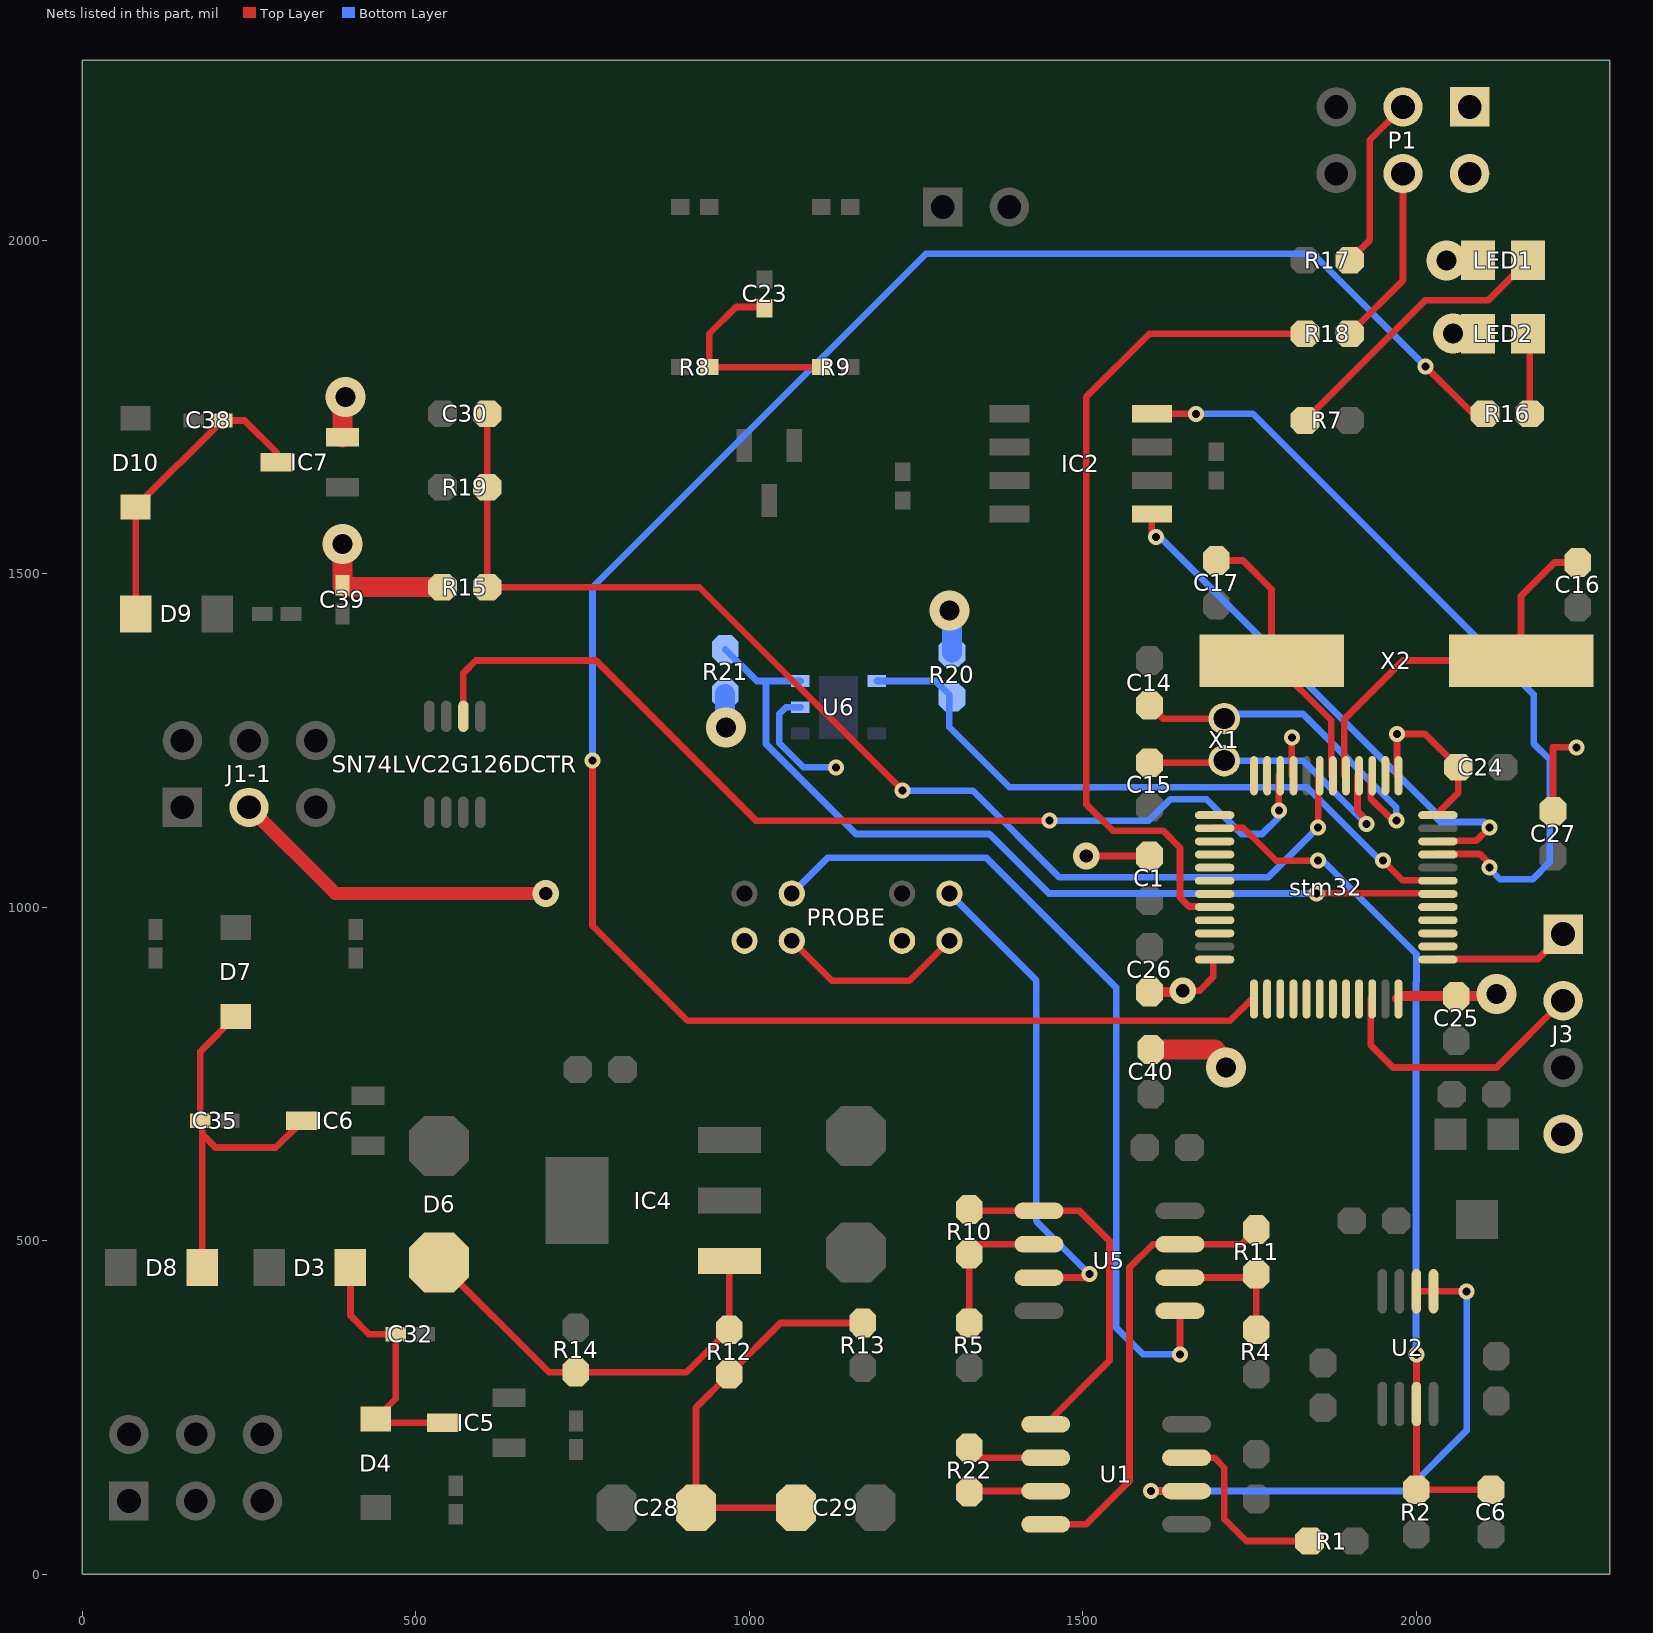
[diagram p0: the nets of this part, all layers, seen from the top]
# Altium PCB MISC82170.PcbDoc (part 2 of 2)
Units mil, origin at the board's own origin, x right, y up, seen from the top; angles counter-clockwise.
Board outline 2290 x 2270 mil, 4 copper layers (Top Layer, GND, VCC, Bottom Layer), stack 43.156 mil thick; 86 components, 73 nets, 279 pads, 92 vias.

## Via types
v1: diameter 60, hole 30, Top Layer to Bottom Layer, 42 vias
v2: diameter 24, hole 12, Top Layer to Bottom Layer, 34 vias
v3: diameter 40, hole 20, Top Layer to Bottom Layer, 16 vias

## Nets (pads, with @x,y where several pads share a name; then routed paths per layer and width w, separated by ;. In a path a pad name is that pad's centre, name@x,y a point inside that pad or via, vN(x,y) a via of type N, cw(c..) or ccw(c..) an arc to the next point about the centre after c; other vN are vias at no path point) (continued)
NetC23_1: C23.1 R8.2 R9.1 | length 318.3
  Top Layer w10: C23.1@1022.89,1898.03 1020.92,1900 980,1900 940,1860 R8.2@940,1810 R9.1@1108.03,1810
NetC28_2: C28.2 C29.2 R12.1 R13.2 | length 602.6
  Top Layer w10: C29.2@1070,100 C28.2@920,100 920,250 R12.1@970,300 1047,377 R13.2@1170,377
NetC32_2: C32.2 D3.2 D4.2 IC5.3 | length 394.8
  Top Layer w10: D3.2@402.05,460 402.05,387.95 430,360 C32.2@470,360 470,263.26 D4.2@440,233.26 445.86,227.4 IC5.3@541.6,227.4
NetC35_2: C35.2 D7.2 D8.2 IC6.3 | length 574.7
  Top Layer w10: D8.2@180,460 180,660 ; D7.2@230,836.74 177.08,783.82 C35.2@177.08,680 180,677.08 180,660 ; IC6.3@330,680 290,640 200,640 180,660
NetC38_2: C38.2 D9.2 D10.2 IC7.3 | length 459.8
  Top Layer w10: D9.2@80,1440 D10.2@80,1600 C38.2@210,1730 243.31,1730 291.6,1681.71 IC7.3@291.6,1667.4
NetD6_1: D6.1 IC4.1 R12.2 R14.1 | length 632.6
  Top Layer w10: D6.1@535,467.5 699.5,303 R14.1@740,303 906,303 R12.2@970,367 IC4.1@970,470
NetLED1_2: LED1.2 R7.1 | length 433.8
  Top Layer w10: R7.1@1833,1730 2013,1910 2107.4,1910 LED1.2@2167.4,1970
NetLED2_2: LED2.2 R16.1 | length 121.1
  Top Layer w10: LED2.2@2167.4,1860 2170,1857.4 R16.1@2170,1740
NetP1_3: P1.3 R17.2 | length 263.1
  Top Layer w10: R17.2@1900,1970 1930,2000 1930,2150 P1.3@1980,2200
NetP1_4: P1.4 R18.2 | length 273.1
  Top Layer w10: R18.2@1900,1860 1980,1940 P1.4@1980,2100
NetPROBE_V1-: PROBE.2 PROBE.6 | length 285.9
  Top Layer w10: PROBE.2@1063.78,950 1123.78,890 1240,890 PROBE.6@1300,950
NetPROBE_V+/V2+: PROBE.5 U5.3 | length 735.5
  Top Layer w10: U5.3@1434.39,445 1505,445 v2(1510,450)
  Bottom Layer w10: PROBE.5@1300,1020.87 1430,890.87 1430,530 v2(1510,450)
NetPROBE_V-/V1+: PROBE.1 U5.5 | length 1275.9
  Top Layer w10: v2(1645.61,330) U5.5@1645.61,395
  Bottom Layer w10: PROBE.1@1063.78,1020.87 1117.13,1074.22 1355.78,1074.22 1550,880 1550,370 1590,330 v2(1645.61,330)
NetR1_1: R1.1 U1.7 | length 281.3
  Top Layer w10: U1.7@1655.61,175 1697.07,175 1712.07,160 1712.07,82.93 1745,50 R1.1@1840,50
NetR4_2: R4.2 R11.2 U5.6 | length 199.5
  Top Layer w10: U5.6@1645.61,445 1755,445 R11.2@1760,450 R4.2@1760,367
NetR5_1: R5.1 R10.2 U5.2 | length 213.6
  Top Layer w10: R5.1@1330,377 R10.2@1330,480 1345,495 U5.2@1434.39,495
NetR10_1: R10.1 U1.1 U5.1 | length 544.1
  Top Layer w10: R10.1@1330,547 1332,545 U5.1@1434.39,545 1495,545 1540,500 1540,320.61 U1.1@1444.39,225
NetR11_1: R11.1 U1.4 U5.7 | length 686.1
  Top Layer w10: U1.4@1444.39,75 1505,75 1570,140 1570,460 1605,495 U5.7@1645.61,495 1738,495 R11.1@1760,517
NetR22_1: R22.1 U1.3 | length 115.2
  Top Layer w10: R22.1@1330,123 1332,125 U1.3@1444.39,125
NetR22_2: R22.2 U1.2 | length 120.6
  Top Layer w10: R22.2@1330,190 1345,175 U1.2@1444.39,175
NetU1_6: U1.6 U2.1 U2.2 | length 848.9
  Top Layer w10: v2(1602,125) U1.6@1655.61,125 ; U2.2@2000.19,424.49 U2.1@2025.79,424.49 v2(2075.51,424.49)
  Bottom Layer w10: v2(1602,125) 1985,125 2075.51,215.51 v2(2075.51,424.49)
NRST: C30.2 R15.1 R19.2 stm32.7 | length 1795.2
  Top Layer w10: C30.2@607,1740 R19.2@607,1630 R15.1@607,1480 925,1480 v2(1230,1175) ; v2(1852.84,1120) stm32.7@1852.84,1198.11
  Bottom Layer w10: v2(1230,1175) 1335,1175 1465,1045 1777.84,1045 v2(1852.84,1120)
OSC32_IN: C14.1 stm32.3 X1.1 | length 546.1
  Top Layer w10: C14.1@1600,1303 1620,1283 X1.1@1712.07,1283 ; stm32.3@1931.58,1198.11 1931.58,1163.42 1965,1130 v2(1970,1130)
  Bottom Layer w10: X1.1@1712.07,1283 1719.07,1290 1830,1290 1970,1150 v2(1970,1130)
OSC32_OUT: C15.1 stm32.4 X1.2 | length 444.1
  Top Layer w10: C15.1@1600,1217 1709.07,1217 X1.2@1712.07,1220 ; stm32.4@1911.89,1198.11 1911.89,1144.68 1925,1131.58 v2(1925,1125)
  Bottom Layer w10: X1.2@1712.07,1220 1830,1220 v2(1925,1125)
OSC_IN: C16.2 stm32.5 X2.1 | length 588
  Top Layer w10: stm32.5@1892.21,1198.11 1892.21,1282.21 1980,1370 X2.1@2157.01,1370 2157.01,1467.01 2207,1517 C16.2@2242,1517
OSC_OUT: C17.2 stm32.6 X2.2 | length 416.8
  Top Layer w10: C17.2@1700,1520 1740,1520 1782.99,1477.01 X2.2@1782.99,1370 1872.52,1280.47 stm32.6@1872.52,1198.11
PA0: SN74LVC2G126DCTR.2 stm32.10 | length 1502.8
  Top Layer w10: SN74LVC2G126DCTR.2@571.38,1286.38 571.38,1351.38 590,1370 770,1370 1010,1130 v2(1450,1130) ; v2(1793.78,1145) stm32.10@1793.78,1198.11
  Bottom Layer w10: v2(1450,1130) 1598.86,1130 1630.86,1162 1685.81,1162 1737.81,1110 1768.78,1110 1793.78,1135 v2(1793.78,1145)
PA1: stm32.11
PA2: stm32.12
PA3: stm32.13
PA4: C6.2 R2.2 stm32.14 U2.7 | length 1299.1
  Top Layer w10: stm32.14@1695.35,1119.37 1740.63,1119.37 1790,1070 v2(1852.84,1070) ; v2@2000,330 v2(2000.19,329.81) U2.7@2000.19,255.51 2000.19,127.19 R2.2@2000,127 C6.2@2112,127
  Bottom Layer w10: v2(1852.84,1070) 1860,1070 2000.19,929.81 2000.19,888.79 1999.5,888.11 1999.5,330.5 v2(2000.19,329.81)
PA5: stm32.15
PA6: stm32.16
PA7: stm32.17
PA8: stm32.29
PA9: stm32.30
PA10: stm32.31
PA15: stm32.38
PB0: stm32.18
PB1: stm32.19
PB2/BOOT1: R18.1 stm32.20 | length 1275
  Top Layer w10: stm32.20@1695.35,1001.26 1659.35,1001.26 1645.61,1015 1645.61,1089.39 1620,1115 1545,1115 1505,1155 1505,1765 1600,1860 R18.1@1833,1860
PB3: stm32.39
PB4: stm32.40
PB5: stm32.41
PB6: R21.1 stm32.42 U6.6 | length 1324.9
  Top Layer w10: v2(1850,1020.87) 1850.08,1020.94 stm32.42@2030,1020.94
  Bottom Layer w10: R21.1@963.78,1387 1011.41,1339.37 1025,1339.37 ; U6.6@1076.67,1339.37 1025,1339.37 ; v2(1850,1020.87) 1449.13,1020.87 1360,1110 1160,1110 1025,1245 1025,1339.37
PB7: R20.1 stm32.43 U6.1 | length 991.4
  Top Layer w10: v2(1950,1070) 1979.37,1040.63 stm32.43@2030,1040.63
  Bottom Layer w10: U6.1@1190.89,1339.37 1279.38,1339.37 1300,1318.75 1300,1270 1390,1180 1836.06,1180 1946.06,1070 v2(1950,1070)
PB8/CANRX: IC2.4 stm32.45 | length 1208.7
  Top Layer w10: IC2.4@1603.54,1740 v2(1670,1740) ; stm32.45@2030,1080 2095.31,1080 2110,1065.31 v2(2110,1060)
  Bottom Layer w10: v2(1670,1740) 1755,1740 2175.9,1319.1 2175.9,1245.89 2200,1221.79 2200,1067.89 2174.14,1042.03 2125.86,1042.03 2110,1057.89 v2(2110,1060)
PB9/CANTX: IC2.1 stm32.46 | length 830.5
  Top Layer w10: IC2.1@1603.54,1590 1603.54,1561.46 v2(1610,1555) ; stm32.46@2050,1100 2030.32,1100 2030,1099.68 2089.68,1099.68 v2(2110,1120)
  Bottom Layer w10: v2(1610,1555) 1615.93,1555 2030,1140.93 2030,1133.86 2035.86,1128 2102,1128 v2(2110,1120)
PB10: stm32.21
PB11: stm32.22
PB12: R16.2 stm32.25 | length 3215.3
  Top Layer w10: v2(765,1220) 765,972.52 907.52,830 1720.95,830 stm32.25@1754.41,863.46 ; v2(2014.01,1810.99) 2085,1740 R16.2@2103,1740
  Bottom Layer w10: v2(765,1220) 765,1480 1265,1980 1845,1980 v2(2014.01,1810.99) v2@2015,1810.99
PB13: stm32.26
PB14: stm32.27
PB15: stm32.28
PC13: stm32.2
SWCLK: J3.1 stm32.37 | length 205.5
  Top Layer w10: stm32.37@2030,922.52 2182.52,922.52 J3.1@2220,960
SWDIO: J3.2 stm32.34 | length 413.7
  Top Layer w10: stm32.34@1931.58,863.46 1931.58,793.42 1965,760 2120,760 J3.2@2220,860
USB_DM: stm32.32
USB_DP: stm32.33
VCC: C24.2 C25.2 C26.1 C27.1 C39.2 C40.2 IC7.2 J3.4 LED1.1 LED2.1 P1.1 P1.2 R15.2 R20.2 R21.2 stm32.1 stm32.9 stm32.24 stm32.36 stm32.48 U6.5 | length 1520.2
  Top Layer w10: v3(1650,875) 1675,875 1695.36,895.36 stm32.24@1695.36,922.52 ; stm32.9@1813.46,1198.11 v2(1813.46,1255) ; stm32.1@1970.95,1198.11 v2(1970.95,1260) 2013,1260 C24.2@2063,1210 2063,1172.05 stm32.48@2030,1139.05 ; C27.1@2205,1144 2205,1240 v2(2240,1240)
  Top Layer w15: C26.1@1600,873 1648,873 v3(1650,875) ; C40.2@1602,787 C40.2@1609,780 ; stm32.36@1970.95,863.46 1974.48,867 C25.2@2060,867 2117,867 v1(2120,870)
  Top Layer w30: v1@390,1540 C39.2@390,1482.92 392.92,1480 R15.2@540,1480 ; IC7.2@390,1704.8 390,1755 v1@395,1760 ; C40.2@1602,787 1698,787 1715,770 v1(1715,760) ; v1(2045,1970) LED1.1@2092.6,1970 ; v1@2053,1865 2058,1860 LED2.1@2092.6,1860
  Bottom Layer w10: U6.5@1076.67,1300 1055,1300 1045,1290 1045,1246.21 1081.21,1210 v2(1130,1210)
  Bottom Layer w30: R21.2@963.78,1320 963.78,1271.22 v1(965,1270) ; v1(1300,1445) 1303.78,1441.22 R20.2@1303.78,1381.97
  other v1: 390,1545 395,1765 2055,1860
Vin: C1.2 J1-1.3 PROBE.3 PROBE.7 | length 593.5
  Top Layer w10: v3(1505,1077) C1.2@1600,1077
  Top Layer w20: J1-1.3@250,1150 379.13,1020.87 v3(695,1020.87)
pads on no net: J1-1.2 J1-1.6 SN74LVC2G126DCTR.3 SN74LVC2G126DCTR.5 SN74LVC2G126DCTR.7 U6.3 U6.4

## Polygon pours and split planes (outlines as drawn)
GND on GND (split plane): 2269.9,20.1 20.1,20.1 20.1,30 20.1,2249.9 2269.9,2249.9
Vin on VCC (split plane): 1544.9,870.1 615.1,870.1 615.1,1124.9 1544.9,1124.9
2Vinput-2 on VCC (split plane): 604.9,705 605.29,703.05 606.4,701.4 608.05,700.29 610,699.9 944.9,699.9 944.9,355.1 740,355.1 738.05,354.71 736.4,353.6 735.29,351.95 734.9,350 734.9,184 735.29,182.05 736.4,180.4 738.05,179.29 740,178.9 741.95,179.29 742.87,179.9 885,179.9 886.95,180.29 888.6,181.4 889.71,183.05 890.1,185 890.1,229.9 1239.9,229.9 1239.9,155.1 630.1,155.1 630.1,270 630.1,505 629.71,506.95 628.6,508.6 626.95,509.71 625,510.1 312.07,510.1 311.82,510.05 308.61,509.8 305.23,508.98 305.1,508.93 305.1,689.9 510,689.9 511.95,690.29 513.6,691.4 514.71,693.05 515.1,695 515.1,830 514.71,831.95 513.6,833.6 511.95,834.71 510,835.1 415.1,835.1 415.1,1030 415.1,1200 414.71,1201.95 413.6,1203.6 411.95,1204.71 410,1205.1 305,1205.1 303.05,1204.71 301.4,1203.6 300.29,1201.95 299.9,1200 299.9,1035.1 200.1,1035.1 200.1,1314.9 604.9,1314.9
5V on VCC (split plane): 1884.9,1512.11 1781.4,1408.6 1746.4,1373.6 1745.29,1371.95 1744.9,1370 1744.9,1065 1745.29,1063.05 1746.4,1061.4 2004.9,802.89 2004.9,715 2005.29,713.05 2006.4,711.4 2051.4,666.4 2106.4,611.4 2108.05,610.29 2110,609.9 2269.9,609.9 2269.9,20.1 1325.1,20.1 1325.1,725 1324.71,726.95 1323.6,728.6 1321.95,729.71 1320,730.1 1120,730.1 1118.05,729.71 1116.4,728.6 1115.29,726.95 1114.9,725 1114.9,565 1115.29,563.05 1116.4,561.4 1118.05,560.29 1120,559.9 1239.9,559.9 1239.9,240.1 885,240.1 883.05,239.71 881.4,238.6 880.29,236.95 879.9,235 879.9,190.1 745.1,190.1 745.1,344.9 950,344.9 951.95,345.29 953.6,346.4 954.71,348.05 955.1,350 955.1,705 954.71,706.95 953.6,708.6 951.95,709.71 950,710.1 615.1,710.1 615.1,859.9 1429.83,859.9 1429.86,859.86 1431.51,858.75 1433.46,858.36 1435.41,858.75 1437.07,859.86 1437.11,859.9 1550,859.9 1551.95,860.29 1553.6,861.4 1554.71,863.05 1555.1,865 1555.1,1130 1554.71,1131.95 1553.6,1133.6 1551.95,1134.71 1550,1135.1 615.1,1135.1 615.1,1314.9 890.45,1314.9 890.45,1230 890.45,1180 890.84,1178.05 891.95,1176.4 893.6,1175.29 895.55,1174.9 1596.9,1174.9 1596.9,1136.69 1595.85,1134.72 1595.17,1132.49 1594.98,1130.58 1594.9,1130.17 1594.9,855 1594.9,850 1594.9,710 1594.9,706.04 1594.97,705.71 1595.2,703.38 1595.97,700.83 1597.23,698.48 1598.71,696.67 1598.9,696.4 1600.55,695.29 1602.5,694.9 1799.51,694.9 1801.46,695.29 1803.11,696.4 1804.22,698.05 1804.61,700 1804.61,702.89 1804.71,703.05 1805.1,705 1805.1,863.46 1804.71,865.41 1803.6,867.07 1744.96,925.72 1744.71,926.95 1743.6,928.6 1685.1,987.11 1685.1,1285 1684.71,1286.95 1683.6,1288.6 1418.6,1553.6 1416.95,1554.71 1415,1555.1 1175.1,1555.1 1175.1,1869.9 1884.9,1869.9
VCC on VCC (split plane): 2269.9,620.1 2112.11,620.1 2058.6,673.6 2015.1,717.11 2015.1,805 2014.71,806.95 2013.6,808.6 1755.1,1067.11 1755.1,1367.89 1788.6,1401.4 1893.6,1506.4 1894.71,1508.05 1895.1,1510 1895.1,1875 1894.71,1876.95 1893.6,1878.6 1891.95,1879.71 1890,1880.1 1170,1880.1 1168.05,1879.71 1166.4,1878.6 1165.29,1876.95 1164.9,1875 1164.9,1550 1165.29,1548.05 1166.4,1546.4 1168.05,1545.29 1170,1544.9 1412.89,1544.9 1674.9,1282.89 1674.9,985 1675.29,983.05 1676.4,981.4 1735.04,922.75 1735.29,921.51 1736.4,919.86 1794.9,861.35 1794.9,721.61 1794.8,721.46 1794.41,719.51 1794.41,705.1 1605.22,705.1 1605.07,705.87 1605.1,706.04 1605.1,710 1605.1,855 1605.1,1130.17 1605.08,1130.25 1605.2,1130.85 1605.54,1131.35 1605.6,1131.4 1606.71,1133.05 1607.1,1135 1607.1,1180 1606.71,1181.95 1605.6,1183.6 1603.95,1184.71 1602,1185.1 900.65,1185.1 900.65,1230 900.65,1318.67 900.54,1319.24 900.37,1320.46 899.68,1322.14 898.93,1323.12 898.6,1323.6 896.95,1324.71 895,1325.1 200.1,1325.1 200.1,1327.89 303.6,1431.4 304.71,1433.05 305.1,1435 305.1,1570 304.71,1571.95 303.6,1573.6 301.95,1574.71 300,1575.1 20.1,1575.1 20.1,2249.9 2269.9,2249.9
2Vinput on VCC (split plane): 404.9,1030 404.9,1025 404.9,830 405.29,828.05 406.4,826.4 408.05,825.29 410,824.9 504.9,824.9 504.9,700.1 305.1,700.1 305.1,710 304.71,711.95 303.6,713.6 301.95,714.71 300,715.1 207.07,715.1 206.88,715.06 204.72,715.27 202.47,715.96 200.39,717.07 200.1,717.31 200.1,1024.9 305,1024.9 306.95,1025.29 308.6,1026.4 309.71,1028.05 310.1,1030 310.1,1194.9 404.9,1194.9
12V on VCC (split plane): 294.9,1437.11 191.4,1333.6 190.29,1331.95 189.9,1330 189.9,715 190.29,713.05 191.4,711.4 191.61,711.25 194.06,709.16 197.02,707.34 200.23,706.02 203.61,705.2 206.82,704.95 207.07,704.9 294.9,704.9 294.9,500 295.29,498.05 296.4,496.4 298.05,495.29 300,494.9 301.95,495.29 303.6,496.4 303.71,496.55 305.39,497.93 307.47,499.04 309.72,499.73 311.88,499.94 312.07,499.9 619.9,499.9 619.9,270 619.9,150 620.29,148.05 621.4,146.4 623.05,145.29 625,144.9 1245,144.9 1246.95,145.29 1248.6,146.4 1249.71,148.05 1250.1,150 1250.1,565 1249.71,566.95 1248.6,568.6 1246.95,569.71 1245,570.1 1125.1,570.1 1125.1,719.9 1314.9,719.9 1314.9,20.1 20.1,20.1 20.1,30 20.1,1564.9 294.9,1564.9

## Keep-outs
Keep-Out Layer:
  lines w10: 0,0 2290,0 2290,2270 0,2270 0,0

## Other copper
VCC (plane layer: these items are gaps in the copper):
  lines w10: 10,1570 300,1570 300,1435 195,1330 195,715 ccw(c207.07,727.07) 207.07,710 300,710 300,500 cw(c312.07,487.93) 312.07,505 625,505 625,270 625,150 1245,150 1245,565 1120,565 1120,725 1320,725 1320,0 ; 195,1030 305,1030 305,1200 410,1200 410,1025 ; 195,1320 610,1320 ; 300,695 510,695 510,830 410,830 410,1030 ; 610,865 1550,865 1550,1130 1530,1130 610,1130 ; 1245,235 885,235 885,185 742.41,185 ccw(c742.41,181.59) 740,184 740,350 950,350 950,705 610,705 610,1320 ; 1433.46,863.46 1435,865 ; 1600,710 1600,706.04 ; 1600,850 1600,1130.17 cw(c1606.83,1130.17) 1602,1135 1602,1180 1480,1180 1445,1180 1095,1180 895.55,1180 895.55,1230 895.55,1318.67 ccw(c893.67,1318.67) 895,1320 610,1320 ; 1600,855 1600,706.04 ; 1800,705 1800,863.46 1740,923.46 1740,925 1680,985 1680,1285 1415,1550 1170,1550 1170,1875 1890,1875 1890,1510 1785,1405 1750,1370 1750,1065 2010,805 2010,715 2055,670 2110,615 2290,615 ; 1800,720 1799.51,719.51 1799.51,700 1755,700 1602.5,700 cw(c1608.54,706.04) 1600,706.04

## Silkscreen, mask and mechanical layers (free items; w line width, h text height)
Bottom Overlay:
  circle w10: c1142.36,1132.36 r393.7
Mechanical 1:
  lines w5.91: 0,0 2290,0 2290,2270 0,2270 0,0